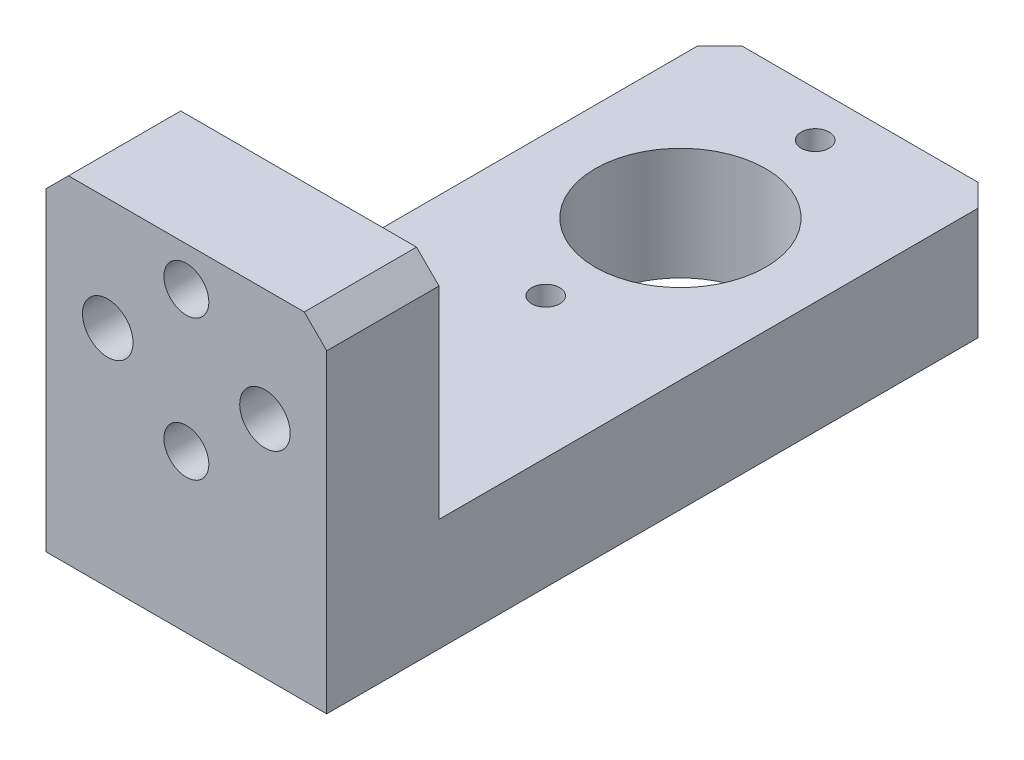
SolidWorks part; units mm, degrees
material "A6061 T6"
ref_plane "前视基准面" through (0, 0, 0) normal (0, 0, 1) x (1, 0, 0)
ref_plane "上视基准面" through (0, 0, 0) normal (0, 1, 0) x (1, 0, 0)
ref_plane "右视基准面" through (0, 0, 0) normal (1, 0, 0) x (0, 0, -1)
sketch "草图1" plane through (0, 0, 0) normal (0, 1, 0) x (1, 0, 0)
  line L1 (-12.5, 30) -> (12.5, 30)
  line L2 (-12.5, 30) -> (-12.5, -30)
  line L3 (-12.5, -30) -> (12.5, -30)
  line L4 (12.5, 30) -> (12.5, -30)
  line L5 (-12.5, 30) -> (12.5, -30) construction
  line L6 (-12.5, -30) -> (12.5, 30) construction
  point P0 (0, 0)
  dimension "D1" = 25
  dimension "D2" = 60
extrude "凸台-拉伸1" add sketch "草图1" along normal blind 10
sketch "草图2" plane through (0, 0, 0) normal (0, -1, 0) x (1, 0, 0)
  line L0 (-12.5, -30) -> (-12.5, 30) construction
  line L1 (12.5, -30) -> (-12.5, -30) construction
  circle A0 centre (0, -14) radius 7.6
  dimension "D1" = 15.2
  dimension "D2" = 12.5
  dimension "D3" = 16
extrude "切除-拉伸1" cut sketch "草图2" against normal blind 20
sketch "草图3" plane through (0, 10, 0) normal (0, 1, 0) x (1, 0, 0)
  line L0 (12.5, -30) -> (12.5, 30) construction
  line L1 (-12.5, -30) -> (12.5, -30)
  line L2 (-12.5, -30) -> (-12.5, -20)
  line L3 (-12.5, -20) -> (12.5, -20)
  line L4 (12.5, -30) -> (12.5, -20)
  dimension "D1" = 10
extrude "凸台-拉伸2" add sketch "草图3" along normal blind 20
chamfer "倒角1" distance 2 angle 45 4 edges at (-12.5, 30, 25) (12.5, 30, 25) (-12.5, 5, -30) (12.5, 5, -30)
hole_wizard "打孔尺寸(%根据)内六角圆柱头螺钉的类型1" positions "草图4" profile "草图5" counterbore size "M4" standard "GB"
sketch "草图4" plane through (0, 0, 20) normal (0, 0, -1) x (-1, 0, 0)
  line L0 (-10.5, 30) -> (10.5, 30) construction
  line L1 (12.5, 28) -> (12.5, 10) construction
  line L2 (-12.5, 28) -> (-12.5, 10) construction
  point P0 (7, 20)
  point P2 (-7, 20)
  dimension "D1" = 10
  dimension "D2" = 5.5
  dimension "D3" = 5.5
sketch "草图5" plane through (-7, 20, 20) normal (1, 0, 0) x (0, 1, 0)
  line L0 (0, 0) -> (0, 16.3519)
  line L1 (0, 16.3519) -> (2.25, 15)
  line L2 (2.25, 15) -> (2.25, 4.6)
  line L3 (2.25, 4.6) -> (4, 4.6)
  line L4 (4, 4.6) -> (4, 0)
  line L5 (4, 0) -> (0, 0)
  line L10 (0, 16.3519) -> (-2.25, 15) construction
  line L11 (0, -6.35) -> (0, 107.95) construction
  dimension "孔直径" = 4.5
  dimension "孔深度" = 15
  dimension "柱形沉头孔直径" = 8
  dimension "柱形沉头孔深度" = 4.6
  dimension "导头角度" = 118
hole_wizard "大小mm 暗销孔1" positions "草图6" profile "草图7" hole size "Ø4.0" standard "GB"
sketch "草图6" plane through (0, 0, 20) normal (0, 0, -1) x (-1, 0, 0)
  line L0 (-10.5, 30) -> (10.5, 30) construction
  line L1 (12.5, 28) -> (12.5, 10) construction
  point P0 (0, 26.5)
  point P2 (0, 14)
  dimension "D1" = 3.5
  dimension "D2" = 12.5
  dimension "D3" = 12.5
sketch "草图7" plane through (0, 26.5, 20) normal (1, 0, 0) x (0, 1, 0)
  line L0 (0, 0) -> (0, 16.2017)
  line L1 (0, 16.2017) -> (2, 15)
  line L2 (2, 15) -> (2, 0)
  line L5 (2, 0) -> (0, 0)
  line L10 (0, 16.2017) -> (-2, 15) construction
  line L11 (0, -6.35) -> (0, 107.95) construction
  dimension "孔直径" = 4
  dimension "孔深度" = 15
  dimension "导头角度" = 118
hole_wizard "M3 螺纹孔1" positions "草图8" profile "草图9" tap size "M3" standard "GB"
sketch "草图8" plane through (0, 0, 0) normal (0, -1, 0) x (-1, 0, 0)
  point P0 (0, 26)
  point P3 (0, 2)
sketch "草图9" plane through (0, 0, -26) normal (1, 0, 0) x (0, 0, -1)
  line L0 (0, 0) -> (0, 15.7511)
  line L1 (0, 15.7511) -> (1.25, 15)
  line L2 (1.25, 15) -> (1.25, 0)
  line L5 (1.25, 0) -> (0, 0)
  line L10 (0, 15.7511) -> (-1.25, 15) construction
  line L11 (0, -6.35) -> (0, 107.95) construction
  dimension "螺纹孔钻头直径" = 2.5
  dimension "螺纹孔钻头深度" = 15
  dimension "导头角度" = 118
cosmetic thread "孔螺蚊线1" parameters "D1"=6, "D2"=3
cosmetic thread "孔螺蚊线2" parameters "D1"=6, "D2"=3
